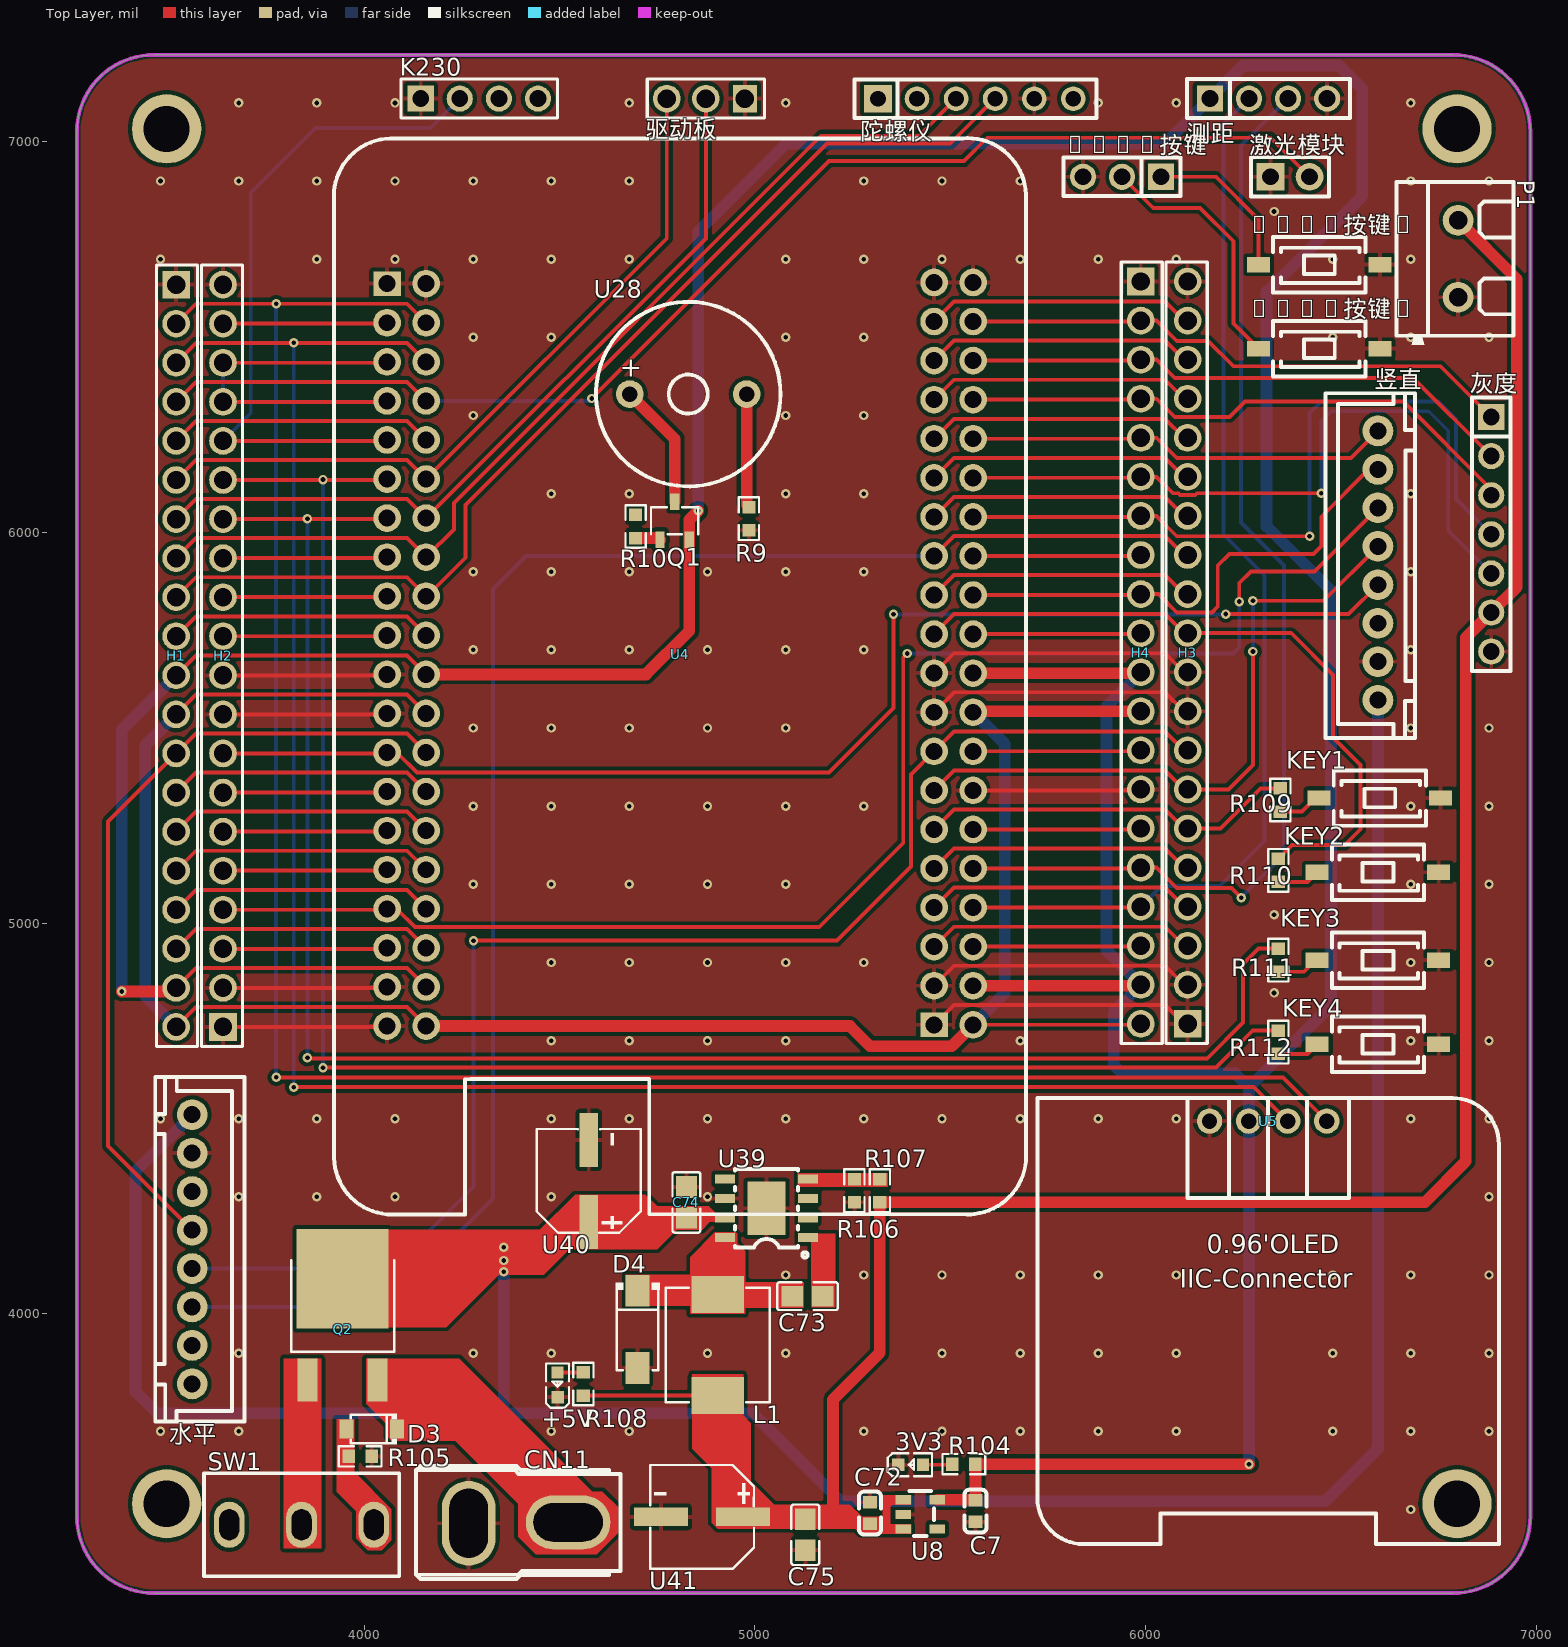
[diagram p0: Top Layer view]
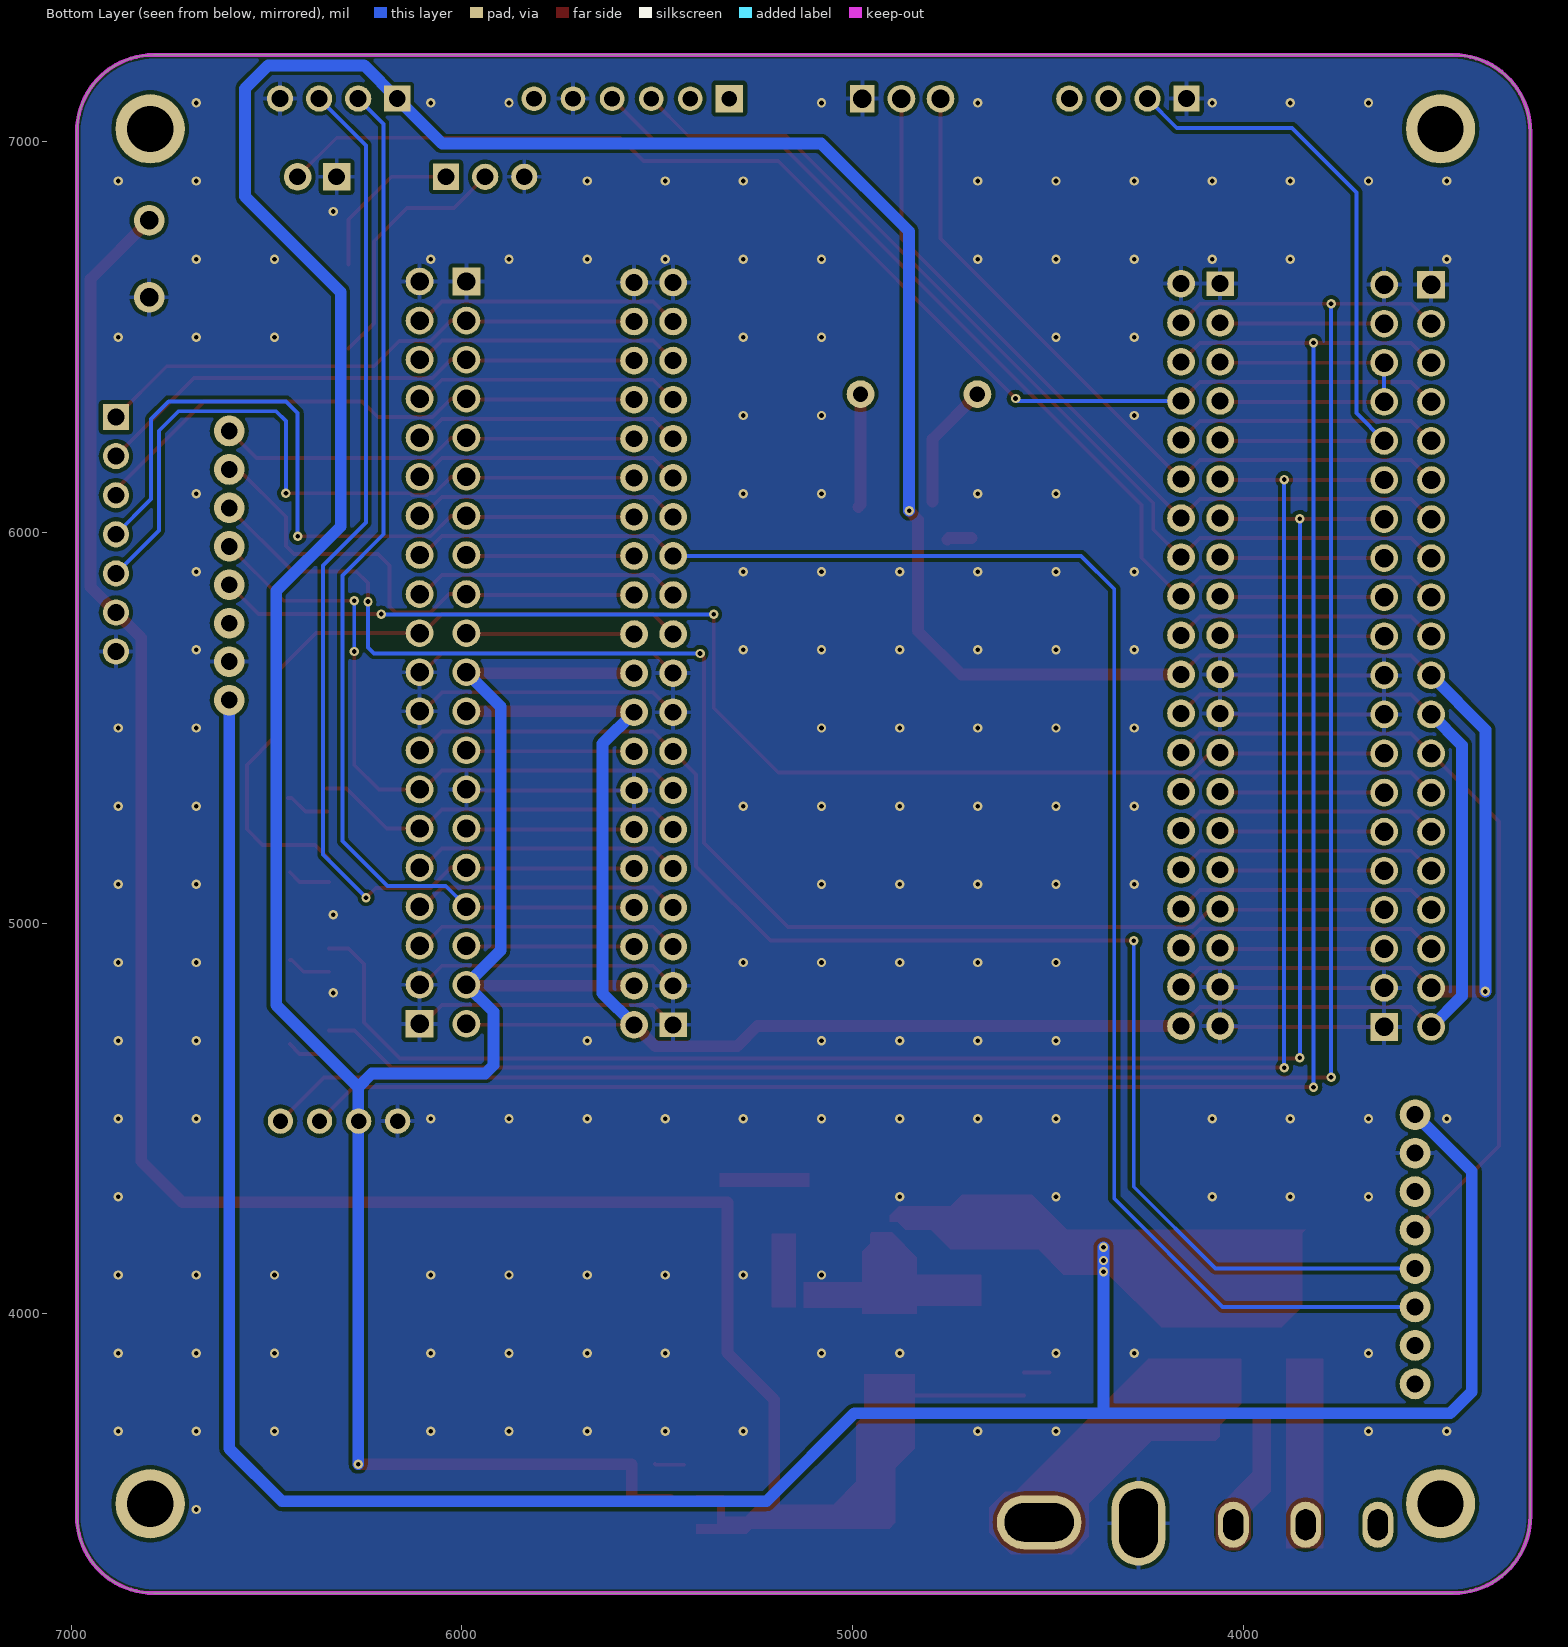
[diagram p1: Bottom Layer view, seen from below]
# Altium PCB MISC49913.pcbdoc
Units mil, origin at the board's own origin, x right, y up, seen from the top; angles counter-clockwise.
Board outline 3720 x 3937 mil, 2 copper layers (Top Layer, Bottom Layer), stack 62.206 mil thick; 52 components, 83 nets, 300 pads, 182 vias.

## Layer stack, top to bottom
Top Solder Mask Layer: solder mask 0.394, Dk 3.3
Top Layer: signal copper 1.379
Dielectric1: surface 59.449, FR4, Dk 4.5
Bottom Layer: signal copper 1.378
Bottom Solder Mask Layer: solder mask 0.394, Dk 3.3

## Board outline
3461.9,7222 ccw(c3461.9,7025.1) 3265,7025.1 3265,3481.9 ccw(c3461.9,3481.9) 3461.9,3285 6788.1,3285 ccw(c6788.1,3481.9) 6985,3481.9 6985,7025.1 ccw(c6788.1,7025.1) 6788.1,7222 3461.9,7222

## Design rules (kind name [scope] priority, off if disabled: settings)
BoardOutlineClearance copperThickness2oz_1 [All] p2 off: genericclearance=7.99 ignorepadtopadclearanceinfootprint=FALSE except(0: Arc-SplitContinuation Track-SplitContinuation SMDPad-SplitContinuation THPad-SplitContinuation Via-SplitContinuation Fill-SplitContinuation Region-SplitContinuation Poly-SplitContinuation Text-SplitContinuation Hole-SplitContinuation; 5.98: Arc-CutoutEdge Track-CutoutEdge SMDPad-CutoutEdge THPad-CutoutEdge Via-CutoutEdge Text-CutoutEdge; 6.9: Hole-OutlineEdge Hole-CutoutEdge; 10: Poly-OutlineEdge Poly-CutoutEdge; 11.81: Arc-OutlineEdge Track-OutlineEdge SMDPad-OutlineEdge THPad-OutlineEdge Via-OutlineEdge Fill-OutlineEdge Region-OutlineEdge Text-OutlineEdge Fill-CutoutEdge Region-CutoutEdge)
BoardOutlineClearance Plane_innerPlane_1 [All] p4 off: genericclearance=4.02 ignorepadtopadclearanceinfootprint=FALSE except(0: Arc-SplitContinuation Track-SplitContinuation SMDPad-SplitContinuation THPad-SplitContinuation Via-SplitContinuation Fill-SplitContinuation Region-SplitContinuation Poly-SplitContinuation Text-SplitContinuation Hole-SplitContinuation; 5.98: Arc-CutoutEdge Track-CutoutEdge SMDPad-CutoutEdge THPad-CutoutEdge Via-CutoutEdge Text-CutoutEdge; 6.9: Hole-OutlineEdge Hole-CutoutEdge; 10: Poly-OutlineEdge Poly-CutoutEdge; 11.81: Arc-OutlineEdge Track-OutlineEdge SMDPad-OutlineEdge THPad-OutlineEdge Via-OutlineEdge Fill-OutlineEdge Region-OutlineEdge Text-OutlineEdge Fill-CutoutEdge Region-CutoutEdge)
BoardOutlineClearance Copper_copperRegion_1 [All] p6 off: genericclearance=4.02 ignorepadtopadclearanceinfootprint=FALSE except(0: Arc-SplitContinuation Track-SplitContinuation SMDPad-SplitContinuation THPad-SplitContinuation Via-SplitContinuation Fill-SplitContinuation Region-SplitContinuation Poly-SplitContinuation Text-SplitContinuation Hole-SplitContinuation; 5.98: Arc-CutoutEdge Track-CutoutEdge SMDPad-CutoutEdge THPad-CutoutEdge Via-CutoutEdge Text-CutoutEdge; 6.9: Hole-OutlineEdge Hole-CutoutEdge; 10: Poly-OutlineEdge Poly-CutoutEdge; 11.81: Arc-OutlineEdge Track-OutlineEdge SMDPad-OutlineEdge THPad-OutlineEdge Via-OutlineEdge Fill-OutlineEdge Region-OutlineEdge Text-OutlineEdge Fill-CutoutEdge Region-CutoutEdge)
BoardOutlineClearance copperThickness1oz_1 [All] p8: genericclearance=4.02 ignorepadtopadclearanceinfootprint=FALSE except(0: Arc-SplitContinuation Track-SplitContinuation SMDPad-SplitContinuation THPad-SplitContinuation Via-SplitContinuation Fill-SplitContinuation Region-SplitContinuation Poly-SplitContinuation Text-SplitContinuation Hole-SplitContinuation; 5.98: Arc-CutoutEdge Track-CutoutEdge SMDPad-CutoutEdge THPad-CutoutEdge Via-CutoutEdge Text-CutoutEdge; 6.9: Hole-OutlineEdge Hole-CutoutEdge; 10: Poly-OutlineEdge Poly-CutoutEdge; 11.81: Arc-OutlineEdge Track-OutlineEdge SMDPad-OutlineEdge THPad-OutlineEdge Via-OutlineEdge Fill-OutlineEdge Region-OutlineEdge Text-OutlineEdge Fill-CutoutEdge Region-CutoutEdge)
Clearance copperThickness2oz [All] p1 off: gap=7.99 ignorepadtopadclearanceinfootprint=FALSE except(5.98: SMDPad-Track SMDPad-SMDPad THPad-Track SMDPad-THPad THPad-THPad Track-Via SMDPad-Via THPad-Via Via-Via Fill-SMDPad Region-SMDPad Fill-THPad Region-THPad Fill-Via Region-Via Fill-Fill Fill-Region Region-Region Arc-Track Arc-SMDPad Arc-THPad Arc-Via Fill-Arc Region-Arc Arc-Arc Text-Track SMDPad-Text Text-THPad Text-Via Fill-Text Region-Text Arc-Text Text-Text; 6.9: Hole-Track Hole-SMDPad Hole-THPad Hole-Via Fill-Hole Region-Hole Hole-Arc Hole-Text; 10: Poly-Track Poly-SMDPad Poly-THPad Poly-Via Poly-Fill Poly-Region Poly-Poly Poly-Arc Poly-Text Poly-Hole; 11.81: Fill-Track Region-Track)
Clearance Plane_innerPlane [All] p3 off: gap=4.02 ignorepadtopadclearanceinfootprint=FALSE except(5.98: SMDPad-Track SMDPad-SMDPad THPad-Track SMDPad-THPad THPad-THPad Track-Via SMDPad-Via THPad-Via Via-Via Fill-SMDPad Region-SMDPad Fill-THPad Region-THPad Fill-Via Region-Via Fill-Fill Fill-Region Region-Region Arc-Track Arc-SMDPad Arc-THPad Arc-Via Fill-Arc Region-Arc Arc-Arc Text-Track SMDPad-Text Text-THPad Text-Via Fill-Text Region-Text Arc-Text Text-Text; 6.9: Hole-Track Hole-SMDPad Hole-THPad Hole-Via Fill-Hole Region-Hole Hole-Arc Hole-Text; 10: Poly-Track Poly-SMDPad Poly-THPad Poly-Via Poly-Fill Poly-Region Poly-Poly Poly-Arc Poly-Text Poly-Hole; 11.81: Fill-Track Region-Track)
Clearance Copper_copperRegion [All] p5 off: gap=4.02 ignorepadtopadclearanceinfootprint=FALSE except(5.98: SMDPad-Track SMDPad-SMDPad THPad-Track SMDPad-THPad THPad-THPad Track-Via SMDPad-Via THPad-Via Via-Via Fill-SMDPad Region-SMDPad Fill-THPad Region-THPad Fill-Via Region-Via Fill-Fill Fill-Region Region-Region Arc-Track Arc-SMDPad Arc-THPad Arc-Via Fill-Arc Region-Arc Arc-Arc Text-Track SMDPad-Text Text-THPad Text-Via Fill-Text Region-Text Arc-Text Text-Text; 6.9: Hole-Track Hole-SMDPad Hole-THPad Hole-Via Fill-Hole Region-Hole Hole-Arc Hole-Text; 10: Poly-Track Poly-SMDPad Poly-THPad Poly-Via Poly-Fill Poly-Region Poly-Poly Poly-Arc Poly-Text Poly-Hole; 11.81: Fill-Track Region-Track)
Clearance copperThickness1oz [All] p7: gap=4.02 ignorepadtopadclearanceinfootprint=FALSE except(5.98: SMDPad-Track SMDPad-SMDPad THPad-Track SMDPad-THPad THPad-THPad Track-Via SMDPad-Via THPad-Via Via-Via Fill-SMDPad Region-SMDPad Fill-THPad Region-THPad Fill-Via Region-Via Fill-Fill Fill-Region Region-Region Arc-Track Arc-SMDPad Arc-THPad Arc-Via Fill-Arc Region-Arc Arc-Arc Text-Track SMDPad-Text Text-THPad Text-Via Fill-Text Region-Text Arc-Text Text-Text; 6.9: Hole-Track Hole-SMDPad Hole-THPad Hole-Via Fill-Hole Region-Hole Hole-Arc Hole-Text; 10: Poly-Track Poly-SMDPad Poly-THPad Poly-Via Poly-Fill Poly-Region Poly-Poly Poly-Arc Poly-Text Poly-Hole; 11.81: Fill-Track Region-Track)
DiffPairsRouting differentialPair [All] p1: maxlimit=6 minlimit=6 mostfreqgap=6 toplayer_minwidth=5 toplayer_prefwidth=10 toplayer_maxwidth=100 toplayer_mingap=6 toplayer_prefgap=6 toplayer_maxgap=6 bottomlayer_minwidth=5 bottomlayer_prefwidth=10 bottomlayer_maxwidth=100 bottomlayer_mingap=6 bottomlayer_prefgap=6 bottomlayer_maxgap=6 maxuncoupledlength=10
HoleToHoleClearance otherClearance [All] p1: gap=11.81 allowstackedmicrovias=TRUE
Length netLength [All] p1: minlimit=0 maxlimit=0
PasteMaskExpansion pasteMaskExpansion [All] p1: expansion=0
PlaneConnect innerPlane [All] p1: planeconnectstyle=Relief reliefexpansion=20 reliefentries=4 reliefconductorwidth=10 reliefairgap=10
PolygonConnect copperRegion [All] p1: connectstyle=Relief reliefconductorwidth=10 reliefentries=4 polygonreliefangle="90 Angle" airgapwidth=10 via.connectstyle=Relief via.reliefconductorwidth=10 via.reliefentries=4 via.polygonreliefangle="90 Angle" via.airgapwidth=10
RoutingVias viaSize [All] p1: holewidth=12.01 width=24.02 viastyle="Through Hole" minholewidth=11.81 minwidth=19.68 maxholewidth=248.03 maxwidth=393.7
SolderMaskExpansion solderMaskExpansion [IsVia] p1: expansion=-1000 istentingtop=TRUE
SolderMaskExpansion solderMaskExpansion [All] p2: expansion=2 istentingtop=FALSE
Width copperThickness2oz_2 [All] p1 off: maxlimit=100 minlimit=8 preferedwidth=10
Width copperThickness1oz_2 [All] p2: maxlimit=100 minlimit=5 preferedwidth=10

## Components (designator, comment, footprint, x,y, rotation, side; value= is the part's Value field where it differs from the comment)
3V3 "" LED_0603 5401.02,3613.64 r0 top
+5V "" LED_0603 4495,3820 r90 top
C7 "1uF" C0603 5565,3495 r90 top
C72 "1uF" C0603 5295,3490 r270 top
C73 "100nF" C0805 5135,4045 r180 top
C74 "100nF" C0805 4825,4285 r270 top
C75 "100nF" C0805 5129.37,3434.37 r90 top
CN11 "AM-1015B-M" CONN-TH_AM-1015B-M 4395,3465 r0 top
D3 "BZT52C16" SOD-123_L2.7-W1.6-LS3.7-RD 4020,3705 r180 top
D4 "SS54" SMA_L4.4-W2.8-LS5.4-R-RD 4700,3960 r270 top
H1 "" HDR-TH_20P-P2.54-V-M-1 3519,5684 r270 top
H2 "" HDR-TH_20P-P2.54-V-M-1 3639,5684 r90 top
H3 "" HDR-TH_20P-P2.54-V-M-1 6108,5692 r90 top
H4 "" HDR-TH_20P-P2.54-V-M-1 5988,5692 r270 top
K230 "2.54*4单排" HDR-TH_4P-P2.54-V-M-1 4295,7110 r0 top
K230按键 "K230按键" HDR-TH_3P-P2.54-V-M 5940,6910 r180 top
K230按键1 "轻触按键3*6*2.5" SW-SMD_L6.0-W3.6-LS8.0 6445,6685 r0 top
K230按键2 "轻触按键3*6*2.5" SW-SMD_L6.0-W3.6-LS8.0 6445,6470 r0 top
KEY1 "轻触按键3*6*2.5" SW-SMD_L6.0-W3.6-LS8.0 6600,5320 r0 top
KEY2 "轻触按键3*6*2.5" SW-SMD_L6.0-W3.6-LS8.0 6595,5130 r0 top
KEY3 "轻触按键3*6*2.5" SW-SMD_L6.0-W3.6-LS8.0 6595,4905 r0 top
KEY4 "轻触按键3*6*2.5" SW-SMD_L6.0-W3.6-LS8.0 6595,4690 r0 top
L1 "4.7uH" IND-SMD_L7.3-W6.6 4905,3920 r90 top
P1 "KF301-2P接线端子" CONN-TH_XY301V-A-5.0-2P 6800,6700 r270 top
Q1 "S8550" SOT-23-3_L2.9-W1.6-P1.90-LS2.8-BR 4795,6030 r270 top
Q2 "HY19P03D" TO-252-2_L6.6-W6.1-P4.57-LS9.9-TL-CW 3945,3960 r90 top
R9 "100Ω" R0603 4985,6035 r90 top
R10 "100Ω" R0603 4695,6015 r90 top
R104 "10K" R0603 5535,3615 r180 top
R105 "10kΩ" R0603 3990,3635 r180 top
R106 "3.24K" R0603 5255,4315 r90 top
R107 "10K" R0603 5320,4315 r270 top
R108 "4.7K" R0603 4561.29,3820.26 r270 top
R109 "100Ω" R0603 6345,5315 r90 top
R110 "100Ω" R0603 6340,5135 r90 top
R111 "100Ω" R0603 6340,4905 r90 top
R112 "100Ω" R0603 6340,4695 r90 top
SW1 "SS-12D10L5" SW-TH_SS-12D10L5 3840,3460 r180 top
U4 "" COMM-TH_LCKFB-TMX-MSPM0G3507 4809,5688 r0 top
U5 "" 0.96OLED_4P 6314,4493 r0 top
U8 "TLV75733PDBVR" SOT-23-5_L2.9-W1.6-P0.95-LS2.8-BL 5423.52,3486.48 r270 top
U28 "2.6kHz" BUZ-TH_BD12.0-P7.60-D0.6-FD 4829.7,6353.8 r0 top
U39 "TPS5430DDAR" ESOP-8_L4.9-W3.9-P1.27-LS6.0-TL-EP 5030,4270 r180 top
U40 "220uF" CAP-SMD_BD6.3-L6.6-W6.6-LS7.2-FD 4575,4340 r90 top
U41 "220uF" CAP-SMD_BD6.3-L6.6-W6.6-LS7.2-FD 4865,3480 r180 top
水平 "水平" CONN-TH_8P-P2.50-XH2.54-8P 3560,4165 r90 top (schematic designator ˮƽ)
测距 "PM2.54-1*4" HDR-TH_4P-P2.54-V-F 6315,7110 r0 top
激光模块 "" HDR-TH_2P-P2.54-V-M-1 6370,6910 r0 top
灰度 "PZ2.54-1*7" HDR-TH_7P-P2.54-V-M 6885,5995 r270 top
竖直 "竖直" CONN-TH_8P-P2.50-XH2.54-8P 6595,5915 r270 top
陀螺仪 "2.54-1*6P母" HDR-TH_6P-P2.54-V-F 5565.21,7110 r0 top
驱动板 "2.54mm-1*3P 直针" HDR-TH_3P-P2.54-V-M-1 4874.68,7110 r180 top

## Footprints (in the part's own frame and the unit in brackets; to place one, negate y for a bottom-side part, rotate by r counter-clockwise, add the part's x,y. Pads: shape width x height; smd on the part's side, far side on the other; paste and mask are expansions set on the pad)
0.96OLED_4P [mm]
  round 1.65 hole 1 copper offset 0,0: 1(-3.81,-0.001) 2(-1.27,0.002) 3(1.27,0.002) 4(3.81,0.002)
  silkscreen extent -15,-27.5 15,1.5
BUZ-TH_BD12.0-P7.60-D0.6-FD [mm]
  round 1.8 hole 1: 1(-3.8,0) 2(3.8,0)
  silkscreen extent -6,-6 6,6
C0603 [mm]
  rect 0.8x0.9 smd: 1(-0.7,0) 2(0.7,0)
  silkscreen extent -1.39,-0.71 1.39,0.71
C0805 [mm]
  rect 1.41x1.35 smd paste-100 mask+0.051: 1(-1,0) 2(1,0)
  silkscreen extent -1.96,-0.9 1.96,0.9
CAP-SMD_BD6.3-L6.6-W6.6-LS7.2-FD [mm]
  rect 3.5x1.2 smd: 1(-2.67,0) 2(2.67,0)
  silkscreen extent -3.38,-3.38 3.38,3.38
COMM-TH_LCKFB-TMX-MSPM0G3507 [mm]
  rect 1.8x1.575 hole 1.1: 1(-19.05,24.09) 41(16.51,-24.09)
  round 1.8 hole 1.1: 2(-16.51,24.09) 3(-19.05,21.55) 4(-16.51,21.55) 5(-19.05,19.01) 6(-16.51,19.01) 7(-19.05,16.47) 8(-16.51,16.47) 9(-19.05,13.93) 10(-16.51,13.93) 11(-19.05,11.39) 12(-16.51,11.39) 13(-19.05,8.85) 14(-16.51,8.85) 15(-19.05,6.31) 16(-16.51,6.31) 17(-19.05,3.77) 18(-16.51,3.77) 19(-19.05,1.23) 20(-16.51,1.23) 21(-19.05,-1.31) 22(-16.51,-1.31) 23(-19.05,-3.85) 24(-16.51,-3.85) 25(-19.05,-6.39) 26(-16.51,-6.39) 27(-19.05,-8.93) 28(-16.51,-8.93) 29(-19.05,-11.47) 30(-16.51,-11.47) 31(-19.05,-14.01) 32(-16.51,-14.01) 33(-19.05,-16.55) 34(-16.51,-16.55) 35(-19.05,-19.09) 36(-16.51,-19.09) 37(-19.05,-21.63) 38(-16.51,-21.63) 39(-19.05,-24.17) 40(-16.51,-24.17) 42(19.05,-24.09) 43(16.51,-21.55) 44(19.05,-21.55) 45(16.51,-19.01) 46(19.05,-19.01) 47(16.51,-16.47) 48(19.05,-16.47) 49(16.51,-13.93) 50(19.05,-13.93) 51(16.51,-11.39) 52(19.05,-11.39) 53(16.51,-8.85) 54(19.05,-8.85) 55(16.51,-6.31) 56(19.05,-6.31) 57(16.51,-3.77) 58(19.05,-3.77) 59(16.51,-1.23) 60(19.05,-1.23) 61(16.51,1.31) 62(19.05,1.31) 63(16.51,3.85) 64(19.05,3.85) 65(16.51,6.39) 66(19.05,6.39) 67(16.51,8.93) 68(19.05,8.93) 69(16.51,11.47) 70(19.05,11.47) 71(16.51,14.01) 72(19.05,14.01) 73(16.51,16.55) 74(19.05,16.55) 75(16.51,19.09) 76(19.05,19.09) 77(16.51,21.63) 78(19.05,21.63) 79(16.51,24.17) 80(19.05,24.17)
  silkscreen extent -22.52,-36.43 22.49,33.55
CONN-TH_8P-P2.50-XH2.54-8P [mm]
  round 2 hole 1.1: 1(8.75,0) 2(6.25,0) 3(3.75,0) 4(1.25,0) 5(-1.25,0) 6(-3.75,0) 7(-6.25,0) 8(-8.75,0)
  silkscreen extent -11.2,-3.4 11.2,2.4
CONN-TH_AM-1015B-M [mm]
  oval 3.5x5.5 hole 2.5 slot 4.5 at 90 deg: 1(-3.231,-0.029)
  oval 5.5x3.5 hole 2.5 slot 4.5 at 0 deg: 2(3.231,0.029)
  silkscreen extent -6.65,-3.65 6.65,3.68
CONN-TH_XY301V-A-5.0-2P [mm]
  round 2 hole 1.2: 1(-2.5,0) 2(2.5,0)
  silkscreen extent -5,-4 5.6,3.6
ESOP-8_L4.9-W3.9-P1.27-LS6.0-TL-EP [mm]
  rect 1.3x0.6 smd: 1(-2.7,1.905) 2(-2.7,0.635) 3(-2.7,-0.635) 4(-2.7,-1.905) 5(2.7,-1.905) 6(2.7,-0.635) 7(2.7,0.635) 8(2.7,1.905)
  rect 2.5x3.5 smd: 9(0,0)
  silkscreen extent -2.67,-2.55 2.05,3.2
HDR-TH_2P-P2.54-V-M-1 [mm]
  rect 1.8x1.8 hole 1.1: 1(-1.27,0)
  round 1.8 hole 1.1: 2(1.27,0)
  silkscreen extent -2.54,-1.27 2.54,1.27
HDR-TH_3P-P2.54-V-M [mm]
  rect 1.7x1.7 hole 1.1: 1(-2.54,0)
  round 1.7 hole 1.1: 2(0,0) 3(2.54,0)
  silkscreen extent -3.81,-1.25 3.81,1.25
HDR-TH_3P-P2.54-V-M-1 [mm]
  rect 1.575x1.8 hole 1.2: 1(-2.54,0)
  round 1.8 hole 1.2: 2(0,0) 3(2.54,0)
  silkscreen extent -3.81,-1.27 3.81,1.27
HDR-TH_4P-P2.54-V-F [mm]
  rect 1.7x1.7 hole 1.1: 1(-3.81,0)
  round 1.7 hole 1.1: 2(-1.27,0) 3(1.27,0) 4(3.81,0)
  silkscreen extent -5.29,-1.27 5.29,1.27
HDR-TH_4P-P2.54-V-M-1 [mm]
  rect 1.7x1.7 hole 1.1: 1(-3.81,0)
  round 1.7 hole 1.1: 2(-1.27,0) 3(1.27,0) 4(3.81,0)
  silkscreen extent -5.08,-1.27 5.08,1.27
HDR-TH_6P-P2.54-V-F [mm]
  rect 1.8x1.8 hole 1.02: 1(-6.35,0)
  round 1.6 hole 1.02: 2(-3.81,0) 3(-1.27,0) 4(1.27,0) 5(3.81,0) 6(6.35,0)
  silkscreen extent -7.87,-1.25 7.87,1.25
HDR-TH_7P-P2.54-V-M [mm]
  rect 1.7x1.7 hole 1.1: 1(-7.62,0)
  round 1.7 hole 1.1: 2(-5.08,0) 3(-2.54,0) 4(0,0) 5(2.54,0) 6(5.08,0) 7(7.62,0)
  silkscreen extent -8.89,-1.25 8.89,1.25
HDR-TH_20P-P2.54-V-M-1 [mm]
  rect 1.8x1.8 hole 1.2: 1(-24.13,0)
  round 1.8 hole 1.2: 2(-21.59,0) 3(-19.05,0) 4(-16.51,0) 5(-13.97,0) 6(-11.43,0) 7(-8.89,0) 8(-6.35,0) 9(-3.81,0) 10(-1.27,0) 11(1.27,0) 12(3.81,0) 13(6.35,0) 14(8.89,0) 15(11.43,0) 16(13.97,0) 17(16.51,0) 18(19.05,0) 19(21.59,0) 20(24.13,0)
  silkscreen extent -25.4,-1.27 25.4,1.4
IND-SMD_L7.3-W6.6 [mm]
  rect 2.424x3.42 smd: 1(3.278,0) 2(-3.278,0)
  silkscreen extent -3.73,-3.38 3.73,3.38
LED_0603 [mil]
  rect 31.5x31.5 smd paste+0 mask+2: 1(-33.5,-0.4) 2(29.5,-0.2)
  silkscreen extent -61,-30 53,30
R0603 [mil]
  rect 31.75x34.02 smd paste-3937.01 mask+2: 1(-29.66,0) 2(29.66,0)
  silkscreen extent -55,-26 55,26
SMA_L4.4-W2.8-LS5.4-R-RD [mil]
  rect 81.2x60.59 smd: 1(98.57,0) 2(-98.57,0)
  silkscreen extent -119,-56 104,56
SOD-123_L2.7-W1.6-LS3.7-RD [mm]
  rect 0.91x1.22 smd: 1(-1.635,0) 2(1.635,0)
  silkscreen extent -1.6,-1 1.38,1
SOT-23-3_L2.9-W1.6-P1.90-LS2.8-BR [mm]
  rect 1.07x0.6 smd: 1(1.235,-0.95) 2(1.235,0.95) 3(-1.235,0)
  silkscreen extent -0.88,-1.54 0.88,1.54
SOT-23-5_L2.9-W1.6-P0.95-LS2.8-BL [mm]
  rect 0.6x1 smd paste+0 mask+0.05: 1(-0.95,-1.1) 2(0,-1.1) 3(0.95,-1.1) 4(0.95,1.1) 5(-0.95,1.1)
  silkscreen extent -1.52,-0.7 1.4,0.89
SW-SMD_L6.0-W3.6-LS8.0 [mm]
  rect 1.5x1 smd: 1(-3.95,0) 2(3.95,0)
  silkscreen extent -3,-1.8 3,1.8
SW-TH_SS-12D10L5 [mm]
  oval 2x3 hole 1.3 slot 2 at 90 deg: 1(-4.7,0) 2(0,0) 3(4.7,0)
  silkscreen extent -6.35,-3.35 6.35,3.35
TO-252-2_L6.6-W6.1-P4.57-LS9.9-TL-CW [mm]
  rect 2.8x1.3 smd: 1(-3.292,2.273) 3(-3.292,-2.273)
  rect 6.5x6 smd: 2(3.292,0)
  silkscreen extent -1.46,-3.35 4.51,3.34

## Free pads (board coordinates)
  round 177.2 hole 118.1: 1(3494.7,7032.7) 2(6797.4,7032.7) 3(3494.7,3513.7) 4(6797.4,3513.7)

## Via types
v1: diameter 24.02, hole 12, Top Layer to Bottom Layer, 182 vias

## Nets (pads, with @x,y where several pads share a name; then routed paths per layer and width w, separated by ;. In a path a pad name is that pad's centre, name@x,y a point inside that pad or via, vN(x,y) a via of type N, cw(c..) or ccw(c..) an arc to the next point about the centre after c; other vN are vias at no path point)
3.3V: 陀螺仪.2
3V3: C7.2 H1.11 H1.19 H4.11 H4.19 Q1.2 R104.1 U4.22 U4.38 U4.44 U4.60 U5.2 U8.5 测距.1 | length 13030.8
  Top Layer w10: H1.19 3570,4885 4110.41,4885 U4.38 ; H1.11 3570,5685 4110.41,5685 U4.22
  Top Layer w30: v1(3380,4825) 3510,4825 H1.19 ; U4.22 4721.41,5636.41 4832.4,5747.4 Q1.2 4832.4,6032.4 v1(4855,6055) ; U8.5 5563.68,3523.88 C7.2 5565,3614.66 R104.1 v1(6265,3615) ; U4.44 5985.59,4839.59 H4.19 ; U4.60 5985.59,5639.59 H4.11
  Bottom Layer w30: v1(3380,4825) 3380,5495 H1.11 ; v1(4855,6055) 4855,6770 5080,6995 6050,6995 测距.1 6250,7195 6495,7195 6555,7135 6555,6860 6310,6615 6310,6015 6475,5850 6475,4790 6265,4580 ; H4.11 5900,5554 5900,4930 H4.19 5918.79,4772.79 5918.79,4636.21 5940,4615 6230,4615 6265,4580 ; U5.2@6264,4493.05 U5.2@6265,4492.05 ; v1(6265,3615) U5.2@6265,4492.05 ; U5.2@6265,4492.05 6265,4580
5V: H1.12 H1.20 H4.12 H4.20 U4.24 U4.40 U4.42 U4.58 | length 5393.4
  Top Layer w10: H1.20 3570,4785 4110.41,4785 U4.40 ; H1.12 3570,5585 4110.41,5585 U4.24 ; U4.42@5579,4739.59 5996.59,4739.59 H4.20@5999,4742 ; H4.12@5996.59,5539.59 H4.12@5999,5542
  Top Layer w30: U4.40 5243.59,4736.41 5295,4685 5504.41,4685 U4.42 ; U4.58 5561.41,5542 H4.12
  Bottom Layer w30: H1.20 3440,4813 3440,5455 H1.12 ; U4.42 5640,4820.59 5640,5458.59 U4.58
12V: C74.2 Q2.2 U39.7 U40.1 水平.1 竖直.1 | length 6462
  Bottom Layer w30: 水平.1 3415,4364.49 3415,3800 3470,3745 4357.33,3745 ; v1(4357.33,4170) v1(4357.33,4136.19) v1(4357.33,4107.32) 4357.33,3745 ; 竖直.1 6595,3655 6460,3520 5220,3520 4995,3745 4357.33,3745
$1N1506: 3V3.2 R104.2 | length 75.5
  Top Layer w10: 3V3.2 5503.78,3613.44 R104.2
$1N2883: H2.11 U4.19 | length 421
  Top Layer w10: H2.11 4056.59,5734 U4.19
$1N2891: H2.3 U4.35 | length 421
  Top Layer w10: H2.3 4056.59,4934 U4.35
$1N2924: H1.18 U4.36 | length 681.3
  Top Layer w10: H1.18 3570,4985 4110.41,4985 U4.36
$1N2927: H1.10 U4.20 | length 681.3
  Top Layer w10: H1.10 3570,5785 4110.41,5785 U4.20
$1N3031: H3.3 U4.45 | length 681.3
  Top Layer w10: U4.45 5510,4990.59 6050.41,4990.59 H3.3@6099,4942
$1N6236: Q1.3 U28.1 | length 322.8
  Top Layer w30: U28.1 4795,6238.9 Q1.3
$1N6238: Q1.1 R10.1 | length 64.2
  Top Layer w30: R10.1 4753.64,5985.34 Q1.1
$1N6240: R9.2 U28.2 | length 291.5
  Top Layer w30: U28.2 4979.31,6070.35 R9.2
$1N19638: CN11.2 D3.1 Q2.3
$1N19825: D3.2 R105.2 SW1.1
$1N19859: Q2.1 SW1.2
$1N23197: C73.1 U39.1
$1N23203: C73.2 D4.2 L1.1 U39.8
$1N23919: +5V.2 R108.1 | length 66.3
  Top Layer w10: +5V.2 4560.86,3849.5 R108.1
$1N33683: KEY1.1 R109.1 | length 113.8
  Top Layer w10: R109.1 6400.34,5285.34 6435,5320 KEY1.1
$1N33684: KEY2.1 R110.1 | length 109.7
  Top Layer w10: R110.1 6414.83,5105.34 KEY2.1
$1N33685: KEY3.1 R111.1 | length 111.8
  Top Layer w10: R111.1 6405.34,4875.34 6435,4905 KEY3.1
$1N33686: KEY4.1 R112.1 | length 109.7
  Top Layer w10: R112.1 6414.83,4665.34 KEY4.1
$1N37357: R106.2 R107.1 U39.4
+5V: C72.2 C75.2 L1.2 P1.1 R107.2 R108.2 U8.1 U8.3 U41.1 灰度.6 | length 5271.6
  Top Layer w10: R108.2 4904.67,3790.61 L1.2
  Top Layer w30: 5200,3475 5200,3780 5320,3900 R107.2 6715.34,4285.34 6820,4390 6820,5730 灰度.6 6950,5860 6950,6648.43 P1.1
BUZZER: R10.2
DIR1: H3.13 U4.65 水平.6 | length 4290.3
  Top Layer w10: U4.65 5510,5990.59 6050.41,5990.59 H3.13@6099,5942
  Bottom Layer w10: 水平.6 4052.36,4017.36 4330,4295 4330,5855 4414.59,5939.59 U4.65
DIR2: H2.4 U4.33 竖直.6 | length 3795.4
  Top Layer w10: H2.4 4056.59,5034 U4.33 4083.59,5036.41 4130,4990 5165,4990 5380,5205 5380,5680 v1(5390,5690) ; v1(6240,5822.8) 6240,5870 6270,5900 6432.36,5900 竖直.6
  Bottom Layer w10: v1(5390,5690) 6225,5690 6240,5705 v1(6240,5822.8)
ECHO: H4.16 U4.50 测距.3 | length 2895.7
  Top Layer w10: U4.50@5579,5139.59 5996.59,5139.59 H4.16@5999,5142 ; H4.16 H4.16@5999,5142 ; v1(6245,5065) 6220,5090 6080,5090 6028,5142 H4.16@5999,5142
  Bottom Layer w10: v1(6245,5065) 6355,5175 6355,5915 6245,6025 6245,6990 测距.3
EN1: H1.13 U4.26 水平.4 | length 2062.2
  Top Layer w10: 水平.4 3345,4429.21 3345,5260 H1.13 3570,5485 4110.41,5485 U4.26
EN2: H2.8 U4.25 竖直.4 | length 3318
  Top Layer w10: H2.8 4056.59,5434 U4.25 4083.59,5436.41 4135,5385 5190,5385 5355,5550 v1(5355,5790) ; v1(6205.79,5790.79) 6520,5790.79 竖直.4
  Bottom Layer w10: v1(5355,5790) 6205,5790 v1(6205.79,5790.79)
GND: 3V3.1 +5V.1 C7.1 C72.1 C74.1 C75.1 CN11.1 D4.1 H1.1 H2.1 H2.2 H2.9 H2.10 H2.20 H3.1 H3.2 H3.9 H3.10 H3.20 H4.1 H4.14 K230.1 K230按键1.2 K230按键2.2 K230按键.3 KEY1.2 KEY2.2 KEY3.2 KEY4.2 P1.2 R9.1 R105.1 R106.1 U4.1 U4.2 U4.21 U4.23 U4.37 U4.39 U4.41 U4.43 U4.54 U4.57 U4.59 U4.79 U4.80 U5.1 U8.2 U39.6 U39.9 U40.2 U41.2 水平.2 测距.4 激光模块.1 灰度.7 竖直.2 陀螺仪.5 驱动板.1 | length 4830
  Top Layer w10: H2.1 4056.59,4734 U4.39 ; H2.2 4056.59,4834 U4.37 ; H2.9 4056.59,5534 U4.23 ; H2.10 4056.59,5634 U4.21 ; U4.41 5510,4790.59 6050.41,4790.59 H3.1@6099,4742 ; U4.43 5510,4890.59 6050.41,4890.59 H3.2@6099,4842 ; U4.57 5510,5590.59 6050.41,5590.59 H3.9@6099,5542 ; U4.59 5510,5690.59 6050.41,5690.59 H3.10@6099,5642 ; U4.54@5579,5339.59 5996.59,5339.59 H4.14@5999,5342
  other v1: 6679.1,3499.1 3479.1,3699.1 3679.1,3699.1 4479.1,3699.1 4679.1,3699.1 5279.1,3699.1 5479.1,3699.1 5679.1,3699.1 5879.1,3699.1 6079.1,3699.1 6479.1,3699.1 6679.1,3699.1 6879.1,3699.1 3679.1,3899.1 4279.1,3899.1 4479.1,3899.1 4879.1,3899.1 5079.1,3899.1 5479.1,3899.1 5679.1,3899.1 5879.1,3899.1 6079.1,3899.1 6479.1,3899.1 6679.1,3899.1 6879.1,3899.1 5079.1,4099.1 5279.1,4099.1 5479.1,4099.1 5679.1,4099.1 5879.1,4099.1 6079.1,4099.1 6479.1,4099.1 6679.1,4099.1 6879.1,4099.1 3679.1,4299.1 3879.1,4299.1 4079.1,4299.1 4479.1,4299.1 4879.1,4299.1 6879.1,4299.1 3479.1,4499.1 3679.1,4499.1 3879.1,4499.1 4079.1,4499.1 4479.1,4499.1 4679.1,4499.1 4879.1,4499.1 5079.1,4499.1 5279.1,4499.1 5479.1,4499.1 5679.1,4499.1 5879.1,4499.1 6079.1,4499.1 6679.1,4499.1 6879.1,4499.1 4479.1,4699.1 4679.1,4699.1 4879.1,4699.1 5079.1,4699.1 5679.1,4699.1 6679.1,4699.1 6879.1,4699.1 6329.1,4821.15 4479.1,4899.1 4679.1,4899.1 4879.1,4899.1 5079.1,4899.1 5279.1,4899.1 6679.1,4899.1 6879.1,4899.1 6329.1,5021.15 4279.1,5099.1 4479.1,5099.1 4679.1,5099.1 4879.1,5099.1 5079.1,5099.1 6679.1,5099.1 6879.1,5099.1 4279.1,5299.1 4479.1,5299.1 4679.1,5299.1 4879.1,5299.1 5079.1,5299.1 5279.1,5299.1 6679.1,5299.1 6879.1,5299.1 4279.1,5499.1 4479.1,5499.1 4679.1,5499.1 4879.1,5499.1 5079.1,5499.1 6679.1,5499.1 6879.1,5499.1 4279.1,5699.1 4479.1,5699.1 4679.1,5699.1 4879.1,5699.1 5079.1,5699.1 5279.1,5699.1 6679.1,5699.1 4279.1,5899.1 4479.1,5899.1 4679.1,5899.1 4879.1,5899.1 5079.1,5899.1 5279.1,5899.1 6679.1,5899.1 4479.1,6099.1 4679.1,6099.1 5079.1,6099.1 5279.1,6099.1 6679.1,6099.1 4279.1,6299.1 5079.1,6299.1 5279.1,6299.1 4279.1,6499.1 4479.1,6499.1 5079.1,6499.1 5279.1,6499.1 6479.1,6499.1 6679.1,6499.1 6879.1,6499.1 3479.1,6699.1 3879.1,6699.1 4079.1,6699.1 4279.1,6699.1 4479.1,6699.1 4679.1,6699.1 5079.1,6699.1 5279.1,6699.1 5479.1,6699.1 5679.1,6699.1 5879.1,6699.1 6079.1,6699.1 6479.1,6699.1 6679.1,6699.1 6329.1,6821.15 3479.1,6899.1 3679.1,6899.1 3879.1,6899.1 4079.1,6899.1 4279.1,6899.1 4479.1,6899.1 4679.1,6899.1 5279.1,6899.1 5479.1,6899.1 5679.1,6899.1 6679.1,6899.1 6879.1,6899.1 3679.1,7099.1 3879.1,7099.1 4079.1,7099.1 4679.1,7099.1 5079.1,7099.1 5879.1,7099.1 6079.1,7099.1 6679.1,7099.1
KEY1: H3.6 R109.2 U4.51 | length 960.8
  Top Layer w10: U4.51 5510,5290.59 6050.41,5290.59 H3.6@6099,5242 ; H3.6 6192,5242 6294.66,5344.66 R109.2
KEY2: H3.11 R110.2 U4.61 | length 1762.8
  Top Layer w10: U4.61 5510,5790.59 6050.41,5790.59 H3.11@6099,5742 ; H3.11 6373,5742 6480,5635 6480,5475 6550,5405 6550,5240 6510,5200 6375.34,5200 R110.2
KEY3: H2.14 R111.2 U4.13 | length 4491.4
  Top Layer w10: H2.14 4056.59,6034 U4.13 ; v1(3855,4655) 3857.01,4652.99 6157.99,4652.99 6250,4745 6250,4895 6289.66,4934.66 R111.2
  Bottom Layer w10: v1(3855,4655) v1(3855,6035)
KEY4: H2.15 R112.2 U4.11 | length 4410.2
  Top Layer w10: H2.15 4056.59,6134 U4.11 ; v1(3895,4630) 6180,4630 6274.66,4724.66 R112.2
  Bottom Layer w10: v1(3895,4630) v1(3895,6135)
KEY5: K230按键1.1 K230按键.1 | length 410.4
  Top Layer w10: K230按键.1 6180,6910 6289.49,6800.51 K230按键1.1
KEY6: K230按键2.1 K230按键.2 | length 655.1
  Top Layer w10: K230按键.2 6020,6830 6140,6830 6225,6745 6225,6534.49 K230按键2.1
OLED_SCL: H1.3 U4.6 U5.3 | length 5166.3
  Top Layer w10: H1.3 3570,6485 v1(3820,6485) 4110.41,6485 U4.6 ; v1(3820,4580) 6277.05,4580 U5.3@6364,4493.05
  Bottom Layer w10: v1(3820,4580) v1(3820,6485)
OLED_SDA: H1.2 U4.4 U5.4 | length 5396.6
  Top Layer w10: H1.2 3570,6585 v1(3775,6585) 4110.41,6585 U4.4 ; v1(3775,4605) 6352.05,4605 U5.4@6464,4493.05
  Bottom Layer w10: v1(3775,4605) v1(3775,6585)
PA0: H2.19 U4.3 | length 421
  Top Layer w10: H2.19 4056.59,6534 U4.3
PA1: H2.17 H2.18 U4.5 U4.7 | length 942
  Top Layer w10: H2.17 4056.59,6334 U4.7 ; H2.18 4056.59,6434 U4.5
  Bottom Layer w10: H2.17 H2.18
PA8: 水平.7
PA9: H2.16 K230.2 U4.9 | length 1720.8
  Top Layer w10: H2.16 4056.59,6234 U4.9
  Bottom Layer w10: H2.16 3710,6305 3710,6870 3875,7035 4170,7035 K230.2
PA10: H1.6 U4.12 驱动板.3 | length 1909.9
  Top Layer w10: H1.6 3570,6185 4110.41,6185 U4.12 4774.68,6752.09 驱动板.3
PA11: H1.7 U4.14 驱动板.2 | length 2051.3
  Top Layer w10: H1.7 3570,6085 4110.41,6085 U4.14 4874.68,6752.09 驱动板.2
PA12: H2.6 U4.29 | length 421
  Top Layer w10: H2.6 4056.59,5234 U4.29
PA13: H1.15 U4.30 | length 681.3
  Top Layer w10: H1.15 3570,5285 4110.41,5285 U4.30
PA14: H3.15 U4.69 | length 681.3
  Top Layer w10: U4.69 5510,6190.59 6050.41,6190.59 H3.15@6099,6142
PA15: H4.6 U4.70 灰度.5 | length 1855.7
  Top Layer w10: U4.70@5579,6139.59 5996.59,6139.59 H4.6@5999,6142 ; H4.6 H4.6@5999,6142 ; v1(6450,6100) 6131.64,6100 6127.23,6095.58 6088.77,6095.58 6084.36,6100 6070,6100 6028,6142 H4.6@5999,6142
  Bottom Layer w10: v1(6450,6100) 6450,6285 6475,6310 6725,6310 6775,6260 6775,6005 灰度.5
PA16: H3.14 U4.67 | length 681.3
  Top Layer w10: U4.67 5510,6090.59 6050.41,6090.59 H3.14@6099,6042
PA17: H4.7 U4.68 灰度.4 | length 1927.9
  Top Layer w10: U4.68@5579,6039.59 5996.59,6039.59 H4.7@5999,6042 ; H4.7 H4.7@5999,6042 ; v1(6420,5990) 6080,5990 6028,6042 H4.7@5999,6042
  Bottom Layer w10: v1(6420,5990) 6420,6305 6450,6335 6750,6335 6795,6290 6795,6085 灰度.4
PA18: H4.18 U4.46 | length 421
  Top Layer w10: U4.46@5579,4939.59 5996.59,4939.59 H4.18@5999,4942
PA21: H4.9 U4.64 竖直.7 | length 1304.5
  Top Layer w10: U4.64@5579,5839.59 5996.59,5839.59 H4.9@5999,5842 ; H4.9 H4.9@5999,5842 ; 竖直.7 6571.06,6161.06 6450,6040 6450,5965 6429.66,5944.66 6214.66,5944.66 6185,5915 6185,5810 6170,5795 6080,5795 6033,5842 H4.9@5999,5842
PA22: H4.5 U4.72 竖直.8 | length 1078.3
  Top Layer w10: U4.72@5579,6239.59 5996.59,6239.59 H4.5@5999,6242 ; H4.5 H4.5@5999,6242 ; 竖直.8 6525.51,6190 6080,6190 6028,6242 H4.5@5999,6242
PA23: H4.10 U4.62 | length 421
  Top Layer w10: U4.62@5579,5739.59 5996.59,5739.59 H4.10@5999,5742
PA24: H4.3 U4.76 灰度.2 | length 1420.3
  Top Layer w10: U4.76@5579,6439.59 5996.59,6439.59 H4.3@5999,6442 ; H4.3 H4.3@5999,6442 ; 灰度.2 6685,6395 6075,6395 6028,6442 H4.3@5999,6442
PA25: H3.18 U4.75 | length 681.3
  Top Layer w10: U4.75 5510,6490.59 6050.41,6490.59 H3.18@6099,6442
PA26: H4.2 U4.78 灰度.1 | length 1420.3
  Top Layer w10: U4.78@5579,6539.59 5996.59,6539.59 H4.2@5999,6542 ; H4.2 H4.2@5999,6542 ; 灰度.1 6755,6425 6225,6425 6160,6490 6080,6490 6028,6542 H4.2@5999,6542
PA27: H3.19 U4.77 | length 681.3
  Top Layer w10: U4.77 5510,6590.59 6050.41,6590.59 H3.19@6099,6542
PA29: H1.17 U4.34 | length 681.3
  Top Layer w10: H1.17 3570,5085 4110.41,5085 U4.34
PA30: H3.7 U4.53 竖直.5 | length 1671.9
  Top Layer w10: U4.53 5510,5390.59 6050.41,5390.59 H3.7@6099,5342 ; H3.7 6212,5342 6275,5405 v1(6275,5695) ; v1(6275,5824.81) 6455.6,5824.81 竖直.5
  Bottom Layer w10: v1(6275,5695) v1(6275,5824.81)
PB1: H4.15 U4.52 | length 421
  Top Layer w10: U4.52@5579,5239.59 5996.59,5239.59 H4.15@5999,5242
PB2: H2.13 U4.15 | length 421
  Top Layer w10: H2.13 4056.59,5934 U4.15
PB3: H2.12 U4.17 | length 421
  Top Layer w10: H2.12 4056.59,5834 U4.17
PB4: H1.4 U4.8 激光模块.2 | length 3262.7
  Top Layer w10: H1.4 3570,6385 4110.41,6385 U4.8 ; v1(4582.5,6342.5) 5190,6950 5535,6950 5595,7010 6320,7010 激光模块.2
  Bottom Layer w10: U4.8 4576.41,6336.41 v1(4582.5,6342.5)
PB5: H1.5 U4.10 | length 681.3
  Top Layer w10: H1.5 3570,6285 4110.41,6285 U4.10
PB8: H2.7 U4.27 | length 421
  Top Layer w10: H2.7 4056.59,5334 U4.27
PB9: H1.14 U4.28 | length 681.3
  Top Layer w10: H1.14 3570,5385 4110.41,5385 U4.28
PB10: H3.5 U4.49 | length 681.3
  Top Layer w10: U4.49 5510,5190.59 6050.41,5190.59 H3.5@6099,5142
PB11: H3.4 U4.47 | length 681.3
  Top Layer w10: U4.47 5510,5090.59 6050.41,5090.59 H3.4@6099,5042
PB12: H1.8 U4.16 陀螺仪.3 | length 2563.2
  Top Layer w10: H1.8 3570,5985 4110.41,5985 U4.16 4230,6007.41 4230,6075 5170,7015 5420.21,7015 陀螺仪.3
PB13: H1.9 U4.18 陀螺仪.4 | length 2744.1
  Top Layer w10: H1.9 3570,5885 4110.41,5885 U4.18 4161.41,5836.41 4260,5935 4260,6070 5185,6995 5500.21,6995 陀螺仪.4
PB14: H4.17 U4.48 测距.2 | length 2778
  Top Layer w10: U4.48@5579,5039.59 5996.59,5039.59 H4.17@5999,5042
  Bottom Layer w10: H4.17 6041,5095 6190,5095 6305,5210 6305,5890 6200,5995 6200,7045 测距.2
PB18: H4.8 U4.66 | length 421
  Top Layer w10: U4.66@5579,5939.59 5996.59,5939.59 H4.8@5999,5942
PB19: H3.12 U4.63 | length 681.3
  Top Layer w10: U4.63 5510,5890.59 6050.41,5890.59 H3.12@6099,5842
PB20: H3.16 U4.71 | length 681.3
  Top Layer w10: U4.71 5510,6290.59 6050.41,6290.59 H3.16@6099,6242
PB21: H3.8 U4.55 水平.5 | length 3635.6
  Top Layer w10: v1(4280,4955) 5210,4955 5400,5145 5400,5380.59 U4.55 5510,5490.59 6050.41,5490.59 H3.8@6099,5442
  Bottom Layer w10: 水平.5 4070.79,4115.79 4280,4325 v1(4280,4955)
PB22: H4.13 U4.56 | length 421
  Top Layer w10: U4.56@5579,5439.59 5996.59,5439.59 H4.13@5999,5442
PB23: H2.5 U4.31 | length 421
  Top Layer w10: H2.5 4056.59,5134 U4.31
PB24: H4.4 U4.74 灰度.3 | length 1462.2
  Top Layer w10: U4.74@5579,6339.59 5996.59,6339.59 H4.4@5999,6342 ; H4.4 H4.4@5999,6342 ; 灰度.3 6885,6110 6660,6335 6255,6335 6215,6295 6075,6295 6028,6342 H4.4@5999,6342
PB25: H3.17 U4.73 | length 681.3
  Top Layer w10: U4.73 5510,6390.59 6050.41,6390.59 H3.17@6099,6342
PB26: H1.16 U4.32 | length 681.3
  Top Layer w10: H1.16 3570,5185 4110.41,5185 U4.32
pads on no net: K230.3 K230.4 SW1.3 U8.4 U39.2 U39.3 U39.5 水平.3 水平.8 竖直.3 陀螺仪.1 陀螺仪.6

## Polygon pours and split planes (outlines as drawn)
GND on Bottom Layer (solid, remove dead copper, pour order 2): 3000,7455 3000,3000 7360,3000 7360,7455
GND on Top Layer (solid, remove dead copper, pour order 0): 3105,7380 3105,3015 7200,3015 7200,7380

## Keep-outs
Board Outline Layer:
  the board outline again, w10

## Other copper
Top Layer:
  region net $1N19859: 3795,3885 3795,3400 3890,3400 3890,3885
  region net $1N19825: 3975,3730 3975,3595 4070,3500 4070,3420 4045,3395 4010,3395 3980.19,3424.81 3980.19,3494.81 3930,3545 3930,3730
  region net $1N19638: 4005,3885 4243.43,3885 4583.43,3545 4610,3545 4650,3505 4650,3440 4595,3385 4439.03,3385 4394.96,3429.08 4394.96,3513.81 4233.77,3675 4070,3675 4060,3685 4060,3715 4005,3770
  region net 12V: 3839.32,4215 4450,4215 4540,4305 4720,4305 4750,4275 4881.71,4275 4905,4251.71 4905,4235 4885,4235 4865,4215 4800,4215 4750,4165 4525,4165 4460,4100 4345,4100 4210,3965 3900.7,3965 3848.34,4017.36 3848.34,4205.98
  region net $1N23203: 4898.08,4208.08 4951.92,4208.08 4955,4205 4955,4180 4975,4160 4975,4000 4835,4000 4835,4145
  region net +5V: 4840,3845 4970,3845 4970,3740 4990,3720 4990,3571.4 5049.73,3511.67 5243.33,3511.67 5274.55,3480.45 5326.45,3480.45 5346.24,3460.67 5400.27,3460.67 5400.27,3436.76 5270.56,3436.76 5257.32,3450 4905,3450 4890,3465 4890,3605 4840,3655
  region net +5V: 5400,3535 5400,3511.67 5351.67,3511.67 5346.24,3506.24 5346.24,3460.67 5327.21,3479.7 5327.21,3532.21 5330,3535
  region net $1N23203: 4670,4100 4670,4020 4925,4020 4925,4100
  region net $1N23203: 4975,4080 4975,4015 5125,4015 5125,4080
  region net $1N23197: 5145,4205 5145,4017.11 5206.31,4017.11 5206.31,4205
  region net $1N37357: 5110,4360 5110,4325 5340,4325 5340,4360